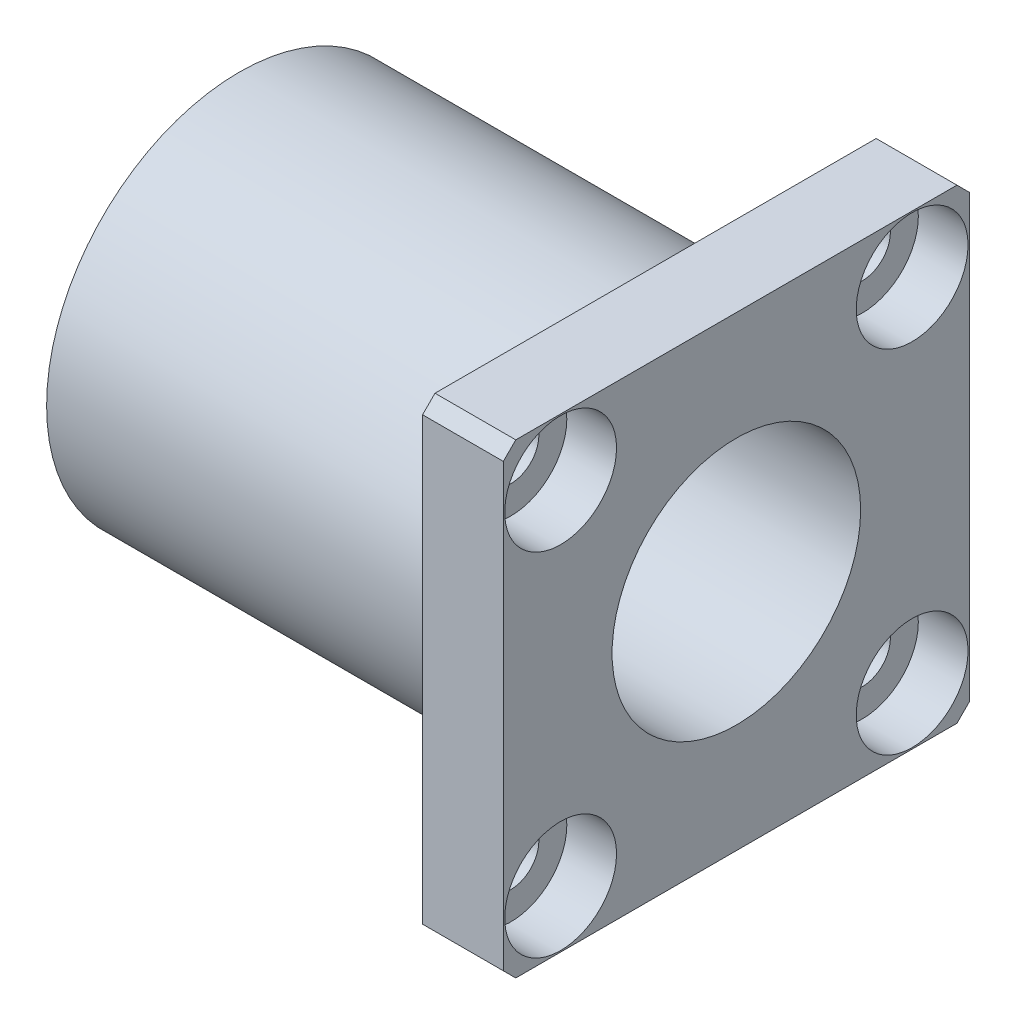
from build123d import *

# Parameters (mm, degrees)
SKETCH1_R                               = 31
SKETCH1_R_2                             = 20
BOSS_EXTRUDE1_DEPTH                     = 67
SKETCH2_W                               = 75
SKETCH2_H                               = 75
SKETCH2_R                               = 20
BOSS_EXTRUDE2_DEPTH                     = 13
CBORE_FOR_M8_HEX_HEAD_BOLT1_D           = 9
CBORE_FOR_M8_HEX_HEAD_BOLT1_CBORE_D     = 18
CBORE_FOR_M8_HEX_HEAD_BOLT1_CBORE_DEPTH = 8
CHAMFER1_SIZE                           = 2


with BuildPart() as part:
    # Sketch1 → Boss-Extrude1 (new body)
    with BuildSketch(Plane(origin=(0, 0, 0), x_dir=(0, 0, -1), z_dir=(1, 0, 0))):
        Circle(SKETCH1_R)
        Circle(SKETCH1_R_2, mode=Mode.SUBTRACT)
    extrude(amount=BOSS_EXTRUDE1_DEPTH)

    # Sketch2 → Boss-Extrude2 (add)
    with BuildSketch(Plane(origin=(67, 0, 0), x_dir=(0, 0, -1), z_dir=(1, 0, 0))):
        Rectangle(SKETCH2_W, SKETCH2_H)
        Circle(SKETCH2_R, mode=Mode.SUBTRACT)
    extrude(amount=BOSS_EXTRUDE2_DEPTH)

    # CBORE for M8 Hex Head Bolt1 (through all)
    with Locations(Plane(origin=(80, 0, 0), x_dir=(0, 0, -1), z_dir=(1, 0, 0))):
        with Locations((28.284271247, 28.284271247), (28.284271247, -28.284271247), (-28.284271247, -28.284271247), (-28.284271247, 28.284271247)):
            CounterBoreHole(CBORE_FOR_M8_HEX_HEAD_BOLT1_D / 2, CBORE_FOR_M8_HEX_HEAD_BOLT1_CBORE_D / 2, CBORE_FOR_M8_HEX_HEAD_BOLT1_CBORE_DEPTH)

    # Chamfer1
    chamfer1_edges = [part.edges().sort_by_distance(p)[0] for p in [
        (73.5, -37.5, -37.5),
        (73.5, 37.5, -37.5),
        (73.5, 37.5, 37.5),
        (73.5, -37.5, 37.5),
    ]]
    chamfer(chamfer1_edges, length=CHAMFER1_SIZE)


solid = part.part
